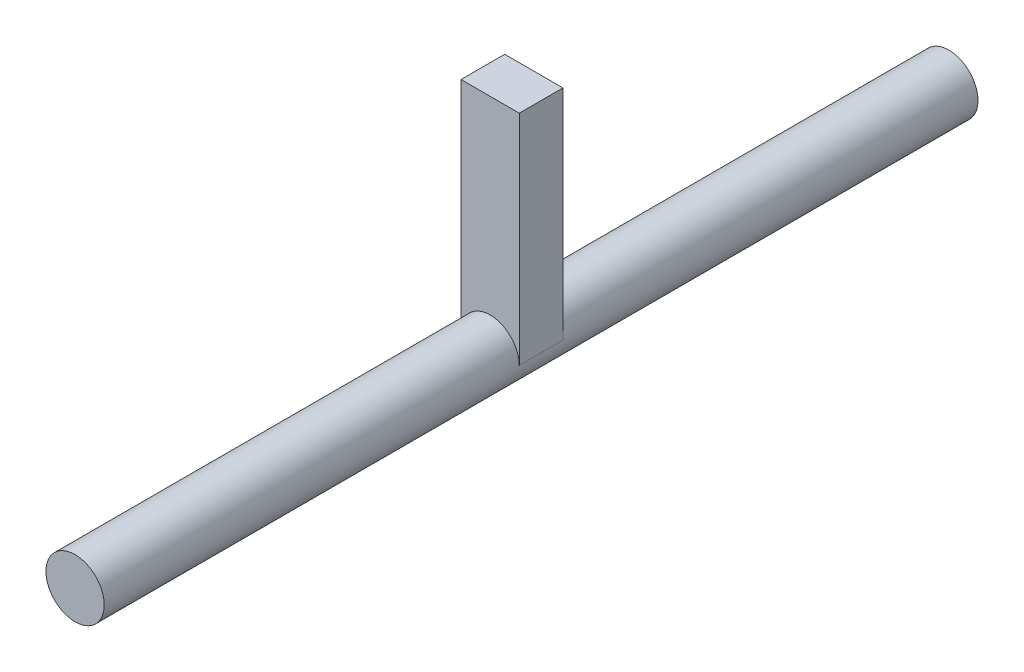
SolidWorks part; units mm, degrees
ref_plane "Front Plane" through (0, 0, 0) normal (0, 0, 1) x (1, 0, 0)
ref_plane "Top Plane" through (0, 0, 0) normal (0, 1, 0) x (1, 0, 0)
ref_plane "Right Plane" through (0, 0, 0) normal (1, 0, 0) x (0, 0, -1)
sketch "Sketch1" plane through (0, 0, 0) normal (0, 0, 1) x (1, 0, 0)
  circle A0 centre (0, 0) radius 4
  dimension "D1" = 8
extrude "Boss-Extrude1" add sketch "Sketch1" along normal blind 120
sketch "Sketch2" plane through (0, 0, 0) normal (0, 1, 0) x (1, 0, 0)
  line L0 (4, -120) -> (4, 0) construction
  line L1 (-4, -57) -> (4, -57)
  line L2 (-4, -57) -> (-4, -63)
  line L3 (-4, -63) -> (4, -63)
  line L4 (4, -57) -> (4, -63)
  line L5 (-4, -57) -> (4, -63) construction
  line L6 (-4, -63) -> (4, -57) construction
  line L7 (-4, -120) -> (4, -120) construction
  point P0 (0, -60)
  dimension "D1" = 6
  dimension "D2" = 60
extrude "Boss-Extrude2" add sketch "Sketch2" along normal blind 30
